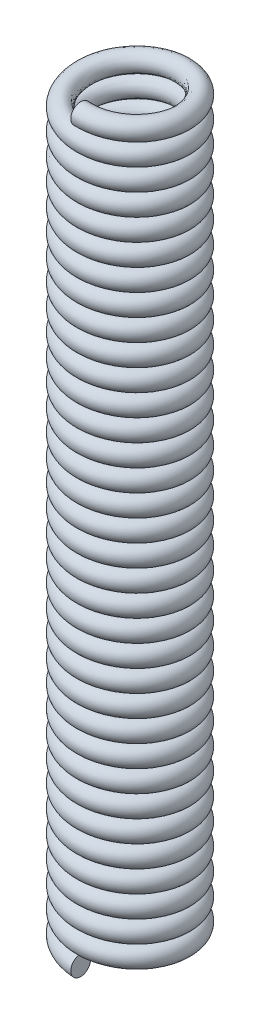
SolidWorks part; units mm, degrees
material "钢"
ref_plane "Front Plane" through (0, 0, 0) normal (0, 0, 1) x (1, 0, 0)
ref_plane "Top Plane" through (0, 0, 0) normal (0, 1, 0) x (1, 0, 0)
ref_plane "Right Plane" through (0, 0, 0) normal (1, 0, 0) x (0, 0, -1)
sketch "Sketch1" plane through (0, 0, 0) normal (0, 1, 0) x (1, 0, 0)
  circle A0 centre (0, 0) radius 1.25
  dimension "D1" = 2.5
curve "Helix/Spiral1" pitch 0.55 height 18.7 turns 34
sketch "Sketch2" plane through (0, 0, 0) normal (1, 0, 0) x (0, 0, -1)
  circle A0 centre (-1.25, 0) radius 0.25
  spline S0 degree 3 poles (-1.25, 0) (-1.25, 0.0114) (-1.1849, 0.0344) (-0.9069, 0.0687) (-0.4908, 0.1031) (0, 0.1375) (0.4908, 0.1719) (0.9069, 0.2062) (1.1849, 0.2406) (1.2825, 0.275) (1.1849, 0.3094) (0.9069, 0.3437) (0.4908, 0.3781) (0, 0.4125) (-0.4908, 0.4469) (-0.9069, 0.4812) (-1.1849, 0.5156) (-1.2825, 0.55) (-1.1849, 0.5844) (-0.9069, 0.6187) (-0.4908, 0.6531) (0, 0.6875) (0.4908, 0.7219) (0.9069, 0.7562) (1.1849, 0.7906) (1.2825, 0.825) (1.1849, 0.8594) (0.9069, 0.8938) (0.4908, 0.9281) (0, 0.9625) (-0.4908, 0.9969) (-0.9069, 1.0312) (-1.1849, 1.0656) (-1.2825, 1.1) (-1.1849, 1.1344) (-0.9069, 1.1687) (-0.4908, 1.2031) (0, 1.2375) (0.4908, 1.2719) (0.9069, 1.3062) (1.1849, 1.3406) (1.2825, 1.375) (1.1849, 1.4094) (0.9069, 1.4437) (0.4908, 1.4781) (0, 1.5125) (-0.4908, 1.5469) (-0.9069, 1.5812) (-1.1849, 1.6156) (-1.2825, 1.65) (-1.1849, 1.6844) (-0.9069, 1.7187) (-0.4908, 1.7531) (0, 1.7875) (0.4908, 1.8219) (0.9069, 1.8562) (1.1849, 1.8906) (1.2825, 1.925) (1.1849, 1.9594) (0.9069, 1.9937) (0.4908, 2.0281) (0, 2.0625) (-0.4908, 2.0969) (-0.9069, 2.1312) (-1.1849, 2.1656) (-1.2825, 2.2) (-1.1849, 2.2344) (-0.9069, 2.2687) (-0.4908, 2.3031) (0, 2.3375) (0.4908, 2.3719) (0.9069, 2.4062) (1.1849, 2.4406) (1.2825, 2.475) (1.1849, 2.5094) (0.9069, 2.5437) (0.4908, 2.5781) (0, 2.6125) (-0.4908, 2.6469) (-0.9069, 2.6813) (-1.1849, 2.7156) (-1.2825, 2.75) (-1.1849, 2.7844) (-0.9069, 2.8188) (-0.4908, 2.8531) (0, 2.8875) (0.4908, 2.9219) (0.9069, 2.9562) (1.1849, 2.9906) (1.2825, 3.025) (1.1849, 3.0594) (0.9069, 3.0938) (0.4908, 3.1281) (0, 3.1625) (-0.4908, 3.1969) (-0.9069, 3.2313) (-1.1849, 3.2656) (-1.2825, 3.3) (-1.1849, 3.3344) (-0.9069, 3.3688) (-0.4908, 3.4031) (0, 3.4375) (0.4908, 3.4719) (0.9069, 3.5063) (1.1849, 3.5406) (1.2825, 3.575) (1.1849, 3.6094) (0.9069, 3.6438) (0.4908, 3.6781) (0, 3.7125) (-0.4908, 3.7469) (-0.9069, 3.7813) (-1.1849, 3.8156) (-1.2825, 3.85) (-1.1849, 3.8844) (-0.9069, 3.9188) (-0.4908, 3.9531) (0, 3.9875) (0.4908, 4.0219) (0.9069, 4.0563) (1.1849, 4.0906) (1.2825, 4.125) (1.1849, 4.1594) (0.9069, 4.1938) (0.4908, 4.2281) (0, 4.2625) (-0.4908, 4.2969) (-0.9069, 4.3312) (-1.1849, 4.3656) (-1.2825, 4.4) (-1.1849, 4.4344) (-0.9069, 4.4688) (-0.4908, 4.5031) (0, 4.5375) (0.4908, 4.5719) (0.9069, 4.6062) (1.1849, 4.6406) (1.2825, 4.675) (1.1849, 4.7094) (0.9069, 4.7437) (0.4908, 4.7781) (0, 4.8125) (-0.4908, 4.8469) (-0.9069, 4.8812) (-1.1849, 4.9156) (-1.2825, 4.95) (-1.1849, 4.9844) (-0.9069, 5.0187) (-0.4908, 5.0531) (0, 5.0875) (0.4908, 5.1219) (0.9069, 5.1562) (1.1849, 5.1906) (1.2825, 5.225) (1.1849, 5.2594) (0.9069, 5.2937) (0.4908, 5.3281) (0, 5.3625) (-0.4908, 5.3969) (-0.9069, 5.4312) (-1.1849, 5.4656) (-1.2825, 5.5) (-1.1849, 5.5344) (-0.9069, 5.5687) (-0.4908, 5.6031) (0, 5.6375) (0.4908, 5.6719) (0.9069, 5.7062) (1.1849, 5.7406) (1.2825, 5.775) (1.1849, 5.8094) (0.9069, 5.8437) (0.4908, 5.8781) (0, 5.9125) (-0.4908, 5.9469) (-0.9069, 5.9812) (-1.1849, 6.0156) (-1.2825, 6.05) (-1.1849, 6.0844) (-0.9069, 6.1187) (-0.4908, 6.1531) (0, 6.1875) (0.4908, 6.2219) (0.9069, 6.2562) (1.1849, 6.2906) (1.2825, 6.325) (1.1849, 6.3594) (0.9069, 6.3937) (0.4908, 6.4281) (0, 6.4625) (-0.4908, 6.4969) (-0.9069, 6.5312) (-1.1849, 6.5656) (-1.2825, 6.6) (-1.1849, 6.6344) (-0.9069, 6.6687) (-0.4908, 6.7031) (0, 6.7375) (0.4908, 6.7719) (0.9069, 6.8062) (1.1849, 6.8406) (1.2825, 6.875) (1.1849, 6.9094) (0.9069, 6.9437) (0.4908, 6.9781) (0, 7.0125) (-0.4908, 7.0469) (-0.9069, 7.0812) (-1.1849, 7.1156) (-1.2825, 7.15) (-1.1849, 7.1844) (-0.9069, 7.2187) (-0.4908, 7.2531) (0, 7.2875) (0.4908, 7.3219) (0.9069, 7.3562) (1.1849, 7.3906) (1.2825, 7.425) (1.1849, 7.4594) (0.9069, 7.4937) (0.4908, 7.5281) (0, 7.5625) (-0.4908, 7.5969) (-0.9069, 7.6312) (-1.1849, 7.6656) (-1.2825, 7.7) (-1.1849, 7.7344) (-0.9069, 7.7687) (-0.4908, 7.8031) (0, 7.8375) (0.4908, 7.8719) (0.9069, 7.9062) (1.1849, 7.9406) (1.2825, 7.975) (1.1849, 8.0094) (0.9069, 8.0437) (0.4908, 8.0781) (0, 8.1125) (-0.4908, 8.1469) (-0.9069, 8.1812) (-1.1849, 8.2156) (-1.2825, 8.25) (-1.1849, 8.2844) (-0.9069, 8.3187) (-0.4908, 8.3531) (0, 8.3875) (0.4908, 8.4219) (0.9069, 8.4562) (1.1849, 8.4906) (1.2825, 8.525) (1.1849, 8.5594) (0.9069, 8.5937) (0.4908, 8.6281) (0, 8.6625) (-0.4908, 8.6969) (-0.9069, 8.7312) (-1.1849, 8.7656) (-1.2825, 8.8) (-1.1849, 8.8344) (-0.9069, 8.8687) (-0.4908, 8.9031) (0, 8.9375) (0.4908, 8.9719) (0.9069, 9.0062) (1.1849, 9.0406) (1.2825, 9.075) (1.1849, 9.1094) (0.9069, 9.1437) (0.4908, 9.1781) (0, 9.2125) (-0.4908, 9.2469) (-0.9069, 9.2812) (-1.1849, 9.3156) (-1.2825, 9.35) (-1.1849, 9.3844) (-0.9069, 9.4187) (-0.4908, 9.4531) (0, 9.4875) (0.4908, 9.5219) (0.9069, 9.5562) (1.1849, 9.5906) (1.2825, 9.625) (1.1849, 9.6594) (0.9069, 9.6937) (0.4908, 9.7281) (0, 9.7625) (-0.4908, 9.7969) (-0.9069, 9.8312) (-1.1849, 9.8656) (-1.2825, 9.9) (-1.1849, 9.9344) (-0.9069, 9.9687) (-0.4908, 10.0031) (0, 10.0375) (0.4908, 10.0719) (0.9069, 10.1062) (1.1849, 10.1406) (1.2825, 10.175) (1.1849, 10.2094) (0.9069, 10.2437) (0.4908, 10.2781) (0, 10.3125) (-0.4908, 10.3469) (-0.9069, 10.3812) (-1.1849, 10.4156) (-1.2825, 10.45) (-1.1849, 10.4844) (-0.9069, 10.5187) (-0.4908, 10.5531) (0, 10.5875) (0.4908, 10.6219) (0.9069, 10.6562) (1.1849, 10.6906) (1.2825, 10.725) (1.1849, 10.7594) (0.9069, 10.7937) (0.4908, 10.8281) (0, 10.8625) (-0.4908, 10.8969) (-0.9069, 10.9312) (-1.1849, 10.9656) (-1.2825, 11) (-1.1849, 11.0344) (-0.9069, 11.0687) (-0.4908, 11.1031) (0, 11.1375) (0.4908, 11.1719) (0.9069, 11.2062) (1.1849, 11.2406) (1.2825, 11.275) (1.1849, 11.3094) (0.9069, 11.3437) (0.4908, 11.3781) (0, 11.4125) (-0.4908, 11.4469) (-0.9069, 11.4812) (-1.1849, 11.5156) (-1.2825, 11.55) (-1.1849, 11.5844) (-0.9069, 11.6187) (-0.4908, 11.6531) (0, 11.6875) (0.4908, 11.7219) (0.9069, 11.7562) (1.1849, 11.7906) (1.2825, 11.825) (1.1849, 11.8594) (0.9069, 11.8937) (0.4908, 11.9281) (0, 11.9625) (-0.4908, 11.9969) (-0.9069, 12.0312) (-1.1849, 12.0656) (-1.2825, 12.1) (-1.1849, 12.1344) (-0.9069, 12.1687) (-0.4908, 12.2031) (0, 12.2375) (0.4908, 12.2719) (0.9069, 12.3062) (1.1849, 12.3406) (1.2825, 12.375) (1.1849, 12.4094) (0.9069, 12.4437) (0.4908, 12.4781) (0, 12.5125) (-0.4908, 12.5469) (-0.9069, 12.5812) (-1.1849, 12.6156) (-1.2825, 12.65) (-1.1849, 12.6844) (-0.9069, 12.7187) (-0.4908, 12.7531) (0, 12.7875) (0.4908, 12.8219) (0.9069, 12.8562) (1.1849, 12.8906) (1.2825, 12.925) (1.1849, 12.9594) (0.9069, 12.9937) (0.4908, 13.0281) (0, 13.0625) (-0.4908, 13.0969) (-0.9069, 13.1312) (-1.1849, 13.1656) (-1.2825, 13.2) (-1.1849, 13.2344) (-0.9069, 13.2687) (-0.4908, 13.3031) (0, 13.3375) (0.4908, 13.3719) (0.9069, 13.4062) (1.1849, 13.4406) (1.2825, 13.475) (1.1849, 13.5094) (0.9069, 13.5437) (0.4908, 13.5781) (0, 13.6125) (-0.4908, 13.6469) (-0.9069, 13.6812) (-1.1849, 13.7156) (-1.2825, 13.75) (-1.1849, 13.7844) (-0.9069, 13.8187) (-0.4908, 13.8531) (0, 13.8875) (0.4908, 13.9219) (0.9069, 13.9562) (1.1849, 13.9906) (1.2825, 14.025) (1.1849, 14.0594) (0.9069, 14.0937) (0.4908, 14.1281) (0, 14.1625) (-0.4908, 14.1969) (-0.9069, 14.2312) (-1.1849, 14.2656) (-1.2825, 14.3) (-1.1849, 14.3344) (-0.9069, 14.3687) (-0.4908, 14.4031) (0, 14.4375) (0.4908, 14.4719) (0.9069, 14.5062) (1.1849, 14.5406) (1.2825, 14.575) (1.1849, 14.6094) (0.9069, 14.6437) (0.4908, 14.6781) (0, 14.7125) (-0.4908, 14.7469) (-0.9069, 14.7812) (-1.1849, 14.8156) (-1.2825, 14.85) (-1.1849, 14.8844) (-0.9069, 14.9187) (-0.4908, 14.9531) (0, 14.9875) (0.4908, 15.0219) (0.9069, 15.0562) (1.1849, 15.0906) (1.2825, 15.125) (1.1849, 15.1594) (0.9069, 15.1937) (0.4908, 15.2281) (0, 15.2625) (-0.4908, 15.2969) (-0.9069, 15.3312) (-1.1849, 15.3656) (-1.2825, 15.4) (-1.1849, 15.4344) (-0.9069, 15.4687) (-0.4908, 15.5031) (0, 15.5375) (0.4908, 15.5719) (0.9069, 15.6062) (1.1849, 15.6406) (1.2825, 15.675) (1.1849, 15.7094) (0.9069, 15.7437) (0.4908, 15.7781) (0, 15.8125) (-0.4908, 15.8469) (-0.9069, 15.8812) (-1.1849, 15.9156) (-1.2825, 15.95) (-1.1849, 15.9844) (-0.9069, 16.0187) (-0.4908, 16.0531) (0, 16.0875) (0.4908, 16.1219) (0.9069, 16.1562) (1.1849, 16.1906) (1.2825, 16.225) (1.1849, 16.2594) (0.9069, 16.2937) (0.4908, 16.3281) (0, 16.3625) (-0.4908, 16.3969) (-0.9069, 16.4312) (-1.1849, 16.4656) (-1.2825, 16.5) (-1.1849, 16.5344) (-0.9069, 16.5687) (-0.4908, 16.6031) (0, 16.6375) (0.4908, 16.6719) (0.9069, 16.7062) (1.1849, 16.7406) (1.2825, 16.775) (1.1849, 16.8094) (0.9069, 16.8437) (0.4908, 16.8781) (0, 16.9125) (-0.4908, 16.9469) (-0.9069, 16.9812) (-1.1849, 17.0156) (-1.2825, 17.05) (-1.1849, 17.0844) (-0.9069, 17.1187) (-0.4908, 17.1531) (0, 17.1875) (0.4908, 17.2219) (0.9069, 17.2562) (1.1849, 17.2906) (1.2825, 17.325) (1.1849, 17.3594) (0.9069, 17.3937) (0.4908, 17.4281) (0, 17.4625) (-0.4908, 17.4969) (-0.9069, 17.5312) (-1.1849, 17.5656) (-1.2825, 17.6) (-1.1849, 17.6344) (-0.9069, 17.6687) (-0.4908, 17.7031) (0, 17.7375) (0.4908, 17.7719) (0.9069, 17.8062) (1.1849, 17.8406) (1.2825, 17.875) (1.1849, 17.9094) (0.9069, 17.9437) (0.4908, 17.9781) (0, 18.0125) (-0.4908, 18.0469) (-0.9069, 18.0812) (-1.1849, 18.1156) (-1.2825, 18.15) (-1.1849, 18.1844) (-0.9069, 18.2188) (-0.4908, 18.2531) (0, 18.2875) (0.4908, 18.3219) (0.9069, 18.3563) (1.1849, 18.3906) (1.2825, 18.425) (1.1849, 18.4594) (0.9069, 18.4938) (0.4908, 18.5281) (0, 18.5625) (-0.4908, 18.5969) (-0.9069, 18.6313) (-1.1849, 18.6656) (-1.25, 18.6886) (-1.25, 18.7) knots 0 0 0 0 0.001838 0.003676 0.005515 0.007353 0.009191 0.011029 0.012868 0.014706 0.016544 0.018382 0.020221 0.022059 0.023897 0.025735 0.027574 0.029412 0.03125 0.033088 0.034926 0.036765 0.038603 0.040441 0.042279 0.044118 0.045956 0.047794 0.049632 0.051471 0.053309 0.055147 0.056985 0.058824 0.060662 0.0625 0.064338 0.066176 0.068015 0.069853 0.071691 0.073529 0.075368 0.077206 0.079044 0.080882 0.082721 0.084559 0.086397 0.088235 0.090074 0.091912 0.09375 0.095588 0.097426 0.099265 0.101103 0.102941 0.104779 0.106618 0.108456 0.110294 0.112132 0.113971 0.115809 0.117647 0.119485 0.121324 0.123162 0.125 0.126838 0.128676 0.130515 0.132353 0.134191 0.136029 0.137868 0.139706 0.141544 0.143382 0.145221 0.147059 0.148897 0.150735 0.152574 0.154412 0.15625 0.158088 0.159926 0.161765 0.163603 0.165441 0.167279 0.169118 0.170956 0.172794 0.174632 0.176471 0.178309 0.180147 0.181985 0.183824 0.185662 0.1875 0.189338 0.191176 0.193015 0.194853 0.196691 0.198529 0.200368 0.202206 0.204044 0.205882 0.207721 0.209559 0.211397 0.213235 0.215074 0.216912 0.21875 0.220588 0.222426 0.224265 0.226103 0.227941 0.229779 0.231618 0.233456 0.235294 0.237132 0.238971 0.240809 0.242647 0.244485 0.246324 0.248162 0.25 0.251838 0.253676 0.255515 0.257353 0.259191 0.261029 0.262868 0.264706 0.266544 0.268382 0.270221 0.272059 0.273897 0.275735 0.277574 0.279412 0.28125 0.283088 0.284926 0.286765 0.288603 0.290441 0.292279 0.294118 0.295956 0.297794 0.299632 0.301471 0.303309 0.305147 0.306985 0.308824 0.310662 0.3125 0.314338 0.316176 0.318015 0.319853 0.321691 0.323529 0.325368 0.327206 0.329044 0.330882 0.332721 0.334559 0.336397 0.338235 0.340074 0.341912 0.34375 0.345588 0.347426 0.349265 0.351103 0.352941 0.354779 0.356618 0.358456 0.360294 0.362132 0.363971 0.365809 0.367647 0.369485 0.371324 0.373162 0.375 0.376838 0.378676 0.380515 0.382353 0.384191 0.386029 0.387868 0.389706 0.391544 0.393382 0.395221 0.397059 0.398897 0.400735 0.402574 0.404412 0.40625 0.408088 0.409926 0.411765 0.413603 0.415441 0.417279 0.419118 0.420956 0.422794 0.424632 0.426471 0.428309 0.430147 0.431985 0.433824 0.435662 0.4375 0.439338 0.441176 0.443015 0.444853 0.446691 0.448529 0.450368 0.452206 0.454044 0.455882 0.457721 0.459559 0.461397 0.463235 0.465074 0.466912 0.46875 0.470588 0.472426 0.474265 0.476103 0.477941 0.479779 0.481618 0.483456 0.485294 0.487132 0.488971 0.490809 0.492647 0.494485 0.496324 0.498162 0.5 0.501838 0.503676 0.505515 0.507353 0.509191 0.511029 0.512868 0.514706 0.516544 0.518382 0.520221 0.522059 0.523897 0.525735 0.527574 0.529412 0.53125 0.533088 0.534926 0.536765 0.538603 0.540441 0.542279 0.544118 0.545956 0.547794 0.549632 0.551471 0.553309 0.555147 0.556985 0.558824 0.560662 0.5625 0.564338 0.566176 0.568015 0.569853 0.571691 0.573529 0.575368 0.577206 0.579044 0.580882 0.582721 0.584559 0.586397 0.588235 0.590074 0.591912 0.59375 0.595588 0.597426 0.599265 0.601103 0.602941 0.604779 0.606618 0.608456 0.610294 0.612132 0.613971 0.615809 0.617647 0.619485 0.621324 0.623162 0.625 0.626838 0.628676 0.630515 0.632353 0.634191 0.636029 0.637868 0.639706 0.641544 0.643382 0.645221 0.647059 0.648897 0.650735 0.652574 0.654412 0.65625 0.658088 0.659926 0.661765 0.663603 0.665441 0.667279 0.669118 0.670956 0.672794 0.674632 0.676471 0.678309 0.680147 0.681985 0.683824 0.685662 0.6875 0.689338 0.691176 0.693015 0.694853 0.696691 0.698529 0.700368 0.702206 0.704044 0.705882 0.707721 0.709559 0.711397 0.713235 0.715074 0.716912 0.71875 0.720588 0.722426 0.724265 0.726103 0.727941 0.729779 0.731618 0.733456 0.735294 0.737132 0.738971 0.740809 0.742647 0.744485 0.746324 0.748162 0.75 0.751838 0.753676 0.755515 0.757353 0.759191 0.761029 0.762868 0.764706 0.766544 0.768382 0.770221 0.772059 0.773897 0.775735 0.777574 0.779412 0.78125 0.783088 0.784926 0.786765 0.788603 0.790441 0.792279 0.794118 0.795956 0.797794 0.799632 0.801471 0.803309 0.805147 0.806985 0.808824 0.810662 0.8125 0.814338 0.816176 0.818015 0.819853 0.821691 0.823529 0.825368 0.827206 0.829044 0.830882 0.832721 0.834559 0.836397 0.838235 0.840074 0.841912 0.84375 0.845588 0.847426 0.849265 0.851103 0.852941 0.854779 0.856618 0.858456 0.860294 0.862132 0.863971 0.865809 0.867647 0.869485 0.871324 0.873162 0.875 0.876838 0.878676 0.880515 0.882353 0.884191 0.886029 0.887868 0.889706 0.891544 0.893382 0.895221 0.897059 0.898897 0.900735 0.902574 0.904412 0.90625 0.908088 0.909926 0.911765 0.913603 0.915441 0.917279 0.919118 0.920956 0.922794 0.924632 0.926471 0.928309 0.930147 0.931985 0.933824 0.935662 0.9375 0.939338 0.941176 0.943015 0.944853 0.946691 0.948529 0.950368 0.952206 0.954044 0.955882 0.957721 0.959559 0.961397 0.963235 0.965074 0.966912 0.96875 0.970588 0.972426 0.974265 0.976103 0.977941 0.979779 0.981618 0.983456 0.985294 0.987132 0.988971 0.990809 0.992647 0.994485 0.996324 0.998162 1 1 1 1 construction
  dimension "D1" = 0.5
sweep "Sweep1" add profiles "Sketch2" path "Helix/Spiral1"
